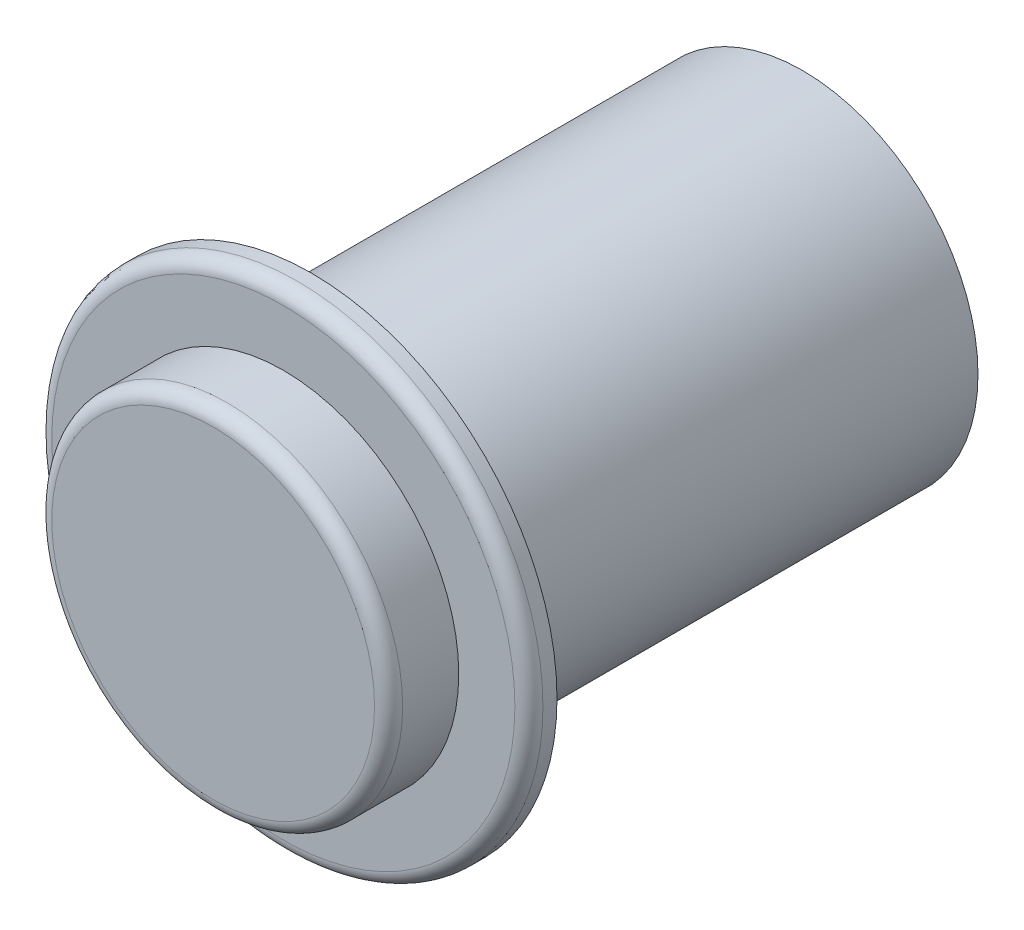
from build123d import *

# Parameters (mm, degrees)
SKETCH1_R           = 12.5
BOSS_EXTRUDE1_DEPTH = 35
SKETCH2_R           = 17.5
BOSS_EXTRUDE2_DEPTH = 2
BOSS_EXTRUDE3_START = 5
SKETCH3_R           = 12.5
BOSS_EXTRUDE3_DEPTH = 5
FILLET1_R           = 1


with BuildPart() as part:
    # Sketch1 → Boss-Extrude1 (new body)
    with BuildSketch(Plane.XY):
        with Locations((336.110854844, 94.216541461)):
            Circle(SKETCH1_R)
    extrude(amount=-BOSS_EXTRUDE1_DEPTH)

    # Sketch2 → Boss-Extrude2 (add)
    with BuildSketch(Plane.XY):
        with Locations((336.110854844, 94.216541461)):
            Circle(SKETCH2_R)
    extrude(amount=BOSS_EXTRUDE2_DEPTH)

    # Sketch3 → Boss-Extrude3 (add)
    with BuildSketch(Plane.XY.offset(2).offset(BOSS_EXTRUDE3_START)):
        with Locations((336.110854844, 94.216541461)):
            Circle(SKETCH3_R)
    extrude(amount=-BOSS_EXTRUDE3_DEPTH)

    # Fillet1
    fillet1_edges = [part.edges().sort_by_distance(p)[0] for p in [
        (323.610854844, 94.216541461, 7),
        (318.610854844, 94.216541461, 2),
    ]]
    fillet(fillet1_edges, radius=FILLET1_R)


solid = part.part
